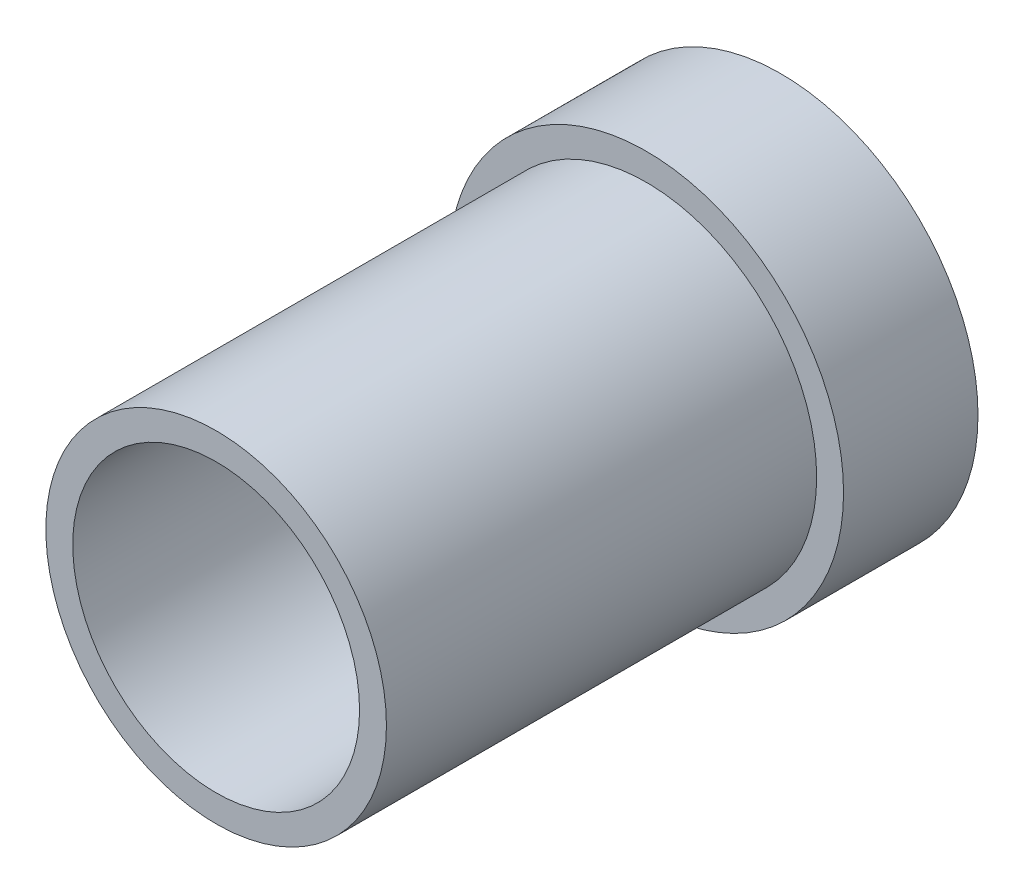
from build123d import *

# Parameters (mm, degrees)
SKETCH_1_R      = 22
SKETCH_1_R_2    = 16
EXTRUDE_1_DEPTH = 15
SKETCH_2_R      = 19
SKETCH_2_R_2    = 16
EXTRUDE_2_DEPTH = 48


with BuildPart() as part:
    # 草图1 → 凸台-拉伸1 (new body)
    with BuildSketch(Plane.XY):
        Circle(SKETCH_1_R)
        Circle(SKETCH_1_R_2, mode=Mode.SUBTRACT)
    extrude(amount=EXTRUDE_1_DEPTH)

    # 草图2 → 凸台-拉伸2 (add)
    with BuildSketch(Plane.XY.offset(15)):
        Circle(SKETCH_2_R)
        Circle(SKETCH_2_R_2, mode=Mode.SUBTRACT)
    extrude(amount=EXTRUDE_2_DEPTH)


solid = part.part
